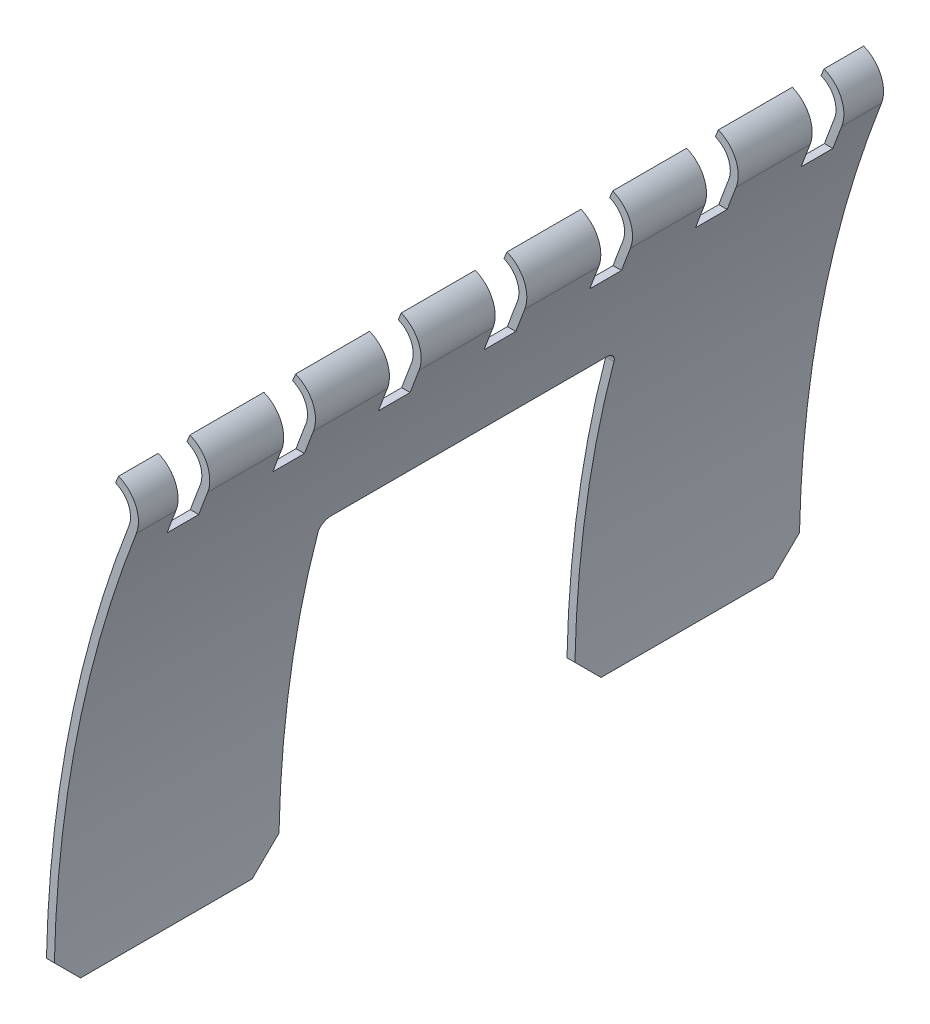
SolidWorks part; units mm, degrees
ref_plane "Front Plane" through (0, 0, 0) normal (0, 0, 1) x (1, 0, 0)
ref_plane "Top Plane" through (0, 0, 0) normal (0, 1, 0) x (1, 0, 0)
ref_plane "Right Plane" through (0, 0, 0) normal (1, 0, 0) x (0, 0, -1)
sketch "Sketch1" plane through (0, 0, 0) normal (0, 0, 1) x (1, 0, 0)
  line L0 (-229.8, 0) -> (-231.3, 0)
  line L1 (0, 0) -> (-315.3117, 122.3014) construction
  arc A0 (-214.248, 83.1013) -> (-229.8, 0) centre (0, 0) ccw
  arc A1 (-215.6465, 83.6438) -> (-231.3, 0) centre (0, 0) ccw
  arc A2 (-217.6012, 90.837) -> (-218.1747, 89.4508) centre (0, 0) ccw
  arc A3 (-214.248, 83.1013) -> (-217.6012, 90.837) centre (-219.842, 85.2711) ccw
  circle A4 centre (0, 0) radius 231.3 construction
  circle A5 centre (0, 0) radius 229.8 construction
  arc A6 (-215.6465, 83.6438) -> (-218.1747, 89.4508) centre (-219.842, 85.2711) ccw
  circle A8 centre (-219.842, 85.2711) radius 4.5 construction
  circle A9 centre (-219.842, 85.2711) radius 6 construction
  point P4 (219.7588, 67.187)
  point P5 (231.3, 0)
  point P8 (-219.842, 85.2711)
  point P19 (-215.342, 85.2711)
  point P21 (-214.1041, 87.0253)
  dimension "D1" = 459.6
  dimension "D4" = 235.8
  dimension "D5" = 12
  dimension "D3" = 21.2
  dimension "D2" = 1.5
extrude "Boss-Extrude1" add sketch "Sketch1" along normal mid plane 141
sketch "Sketch2" plane through (0, 0, 0) normal (0, 0, 1) x (1, 0, 0)
  line L0 (-231.3, 0) -> (-229.8, 0) construction
  line L1 (-256.8852, 60) -> (-194.6945, 60)
  line L2 (-256.8852, 60) -> (-256.8852, -22.2291)
  line L3 (-256.8852, -22.2291) -> (-194.6945, -22.2291)
  line L4 (-194.6945, 60) -> (-194.6945, -22.2291)
  dimension "D1" = 60
extrude "Cut-Extrude1" cut sketch "Sketch2" against normal mid plane 56
fillet "Fillet1" radius 2 2 edges at (-222.6056, 60, 28) (-222.6056, 60, -28)
chamfer "Chamfer2" distance 5 angle 45 4 edges at (-230.55, 0, -28) (-230.55, 0, -70.5) (-230.55, 0, 70.5) (-230.55, 0, 28)
sketch "Sketch3" plane through (0, 0, 0) normal (1, 0, 0) x (0, 0, -1)
  line L0 (70.5, 5) -> (70.5, 83.1013) construction
  line L1 (57, 90.837) -> (63, 90.837)
  line L2 (57, 90.837) -> (57, 78.637)
  line L3 (57, 78.637) -> (63, 78.637)
  line L4 (63, 90.837) -> (63, 78.637)
  line L5 (-70.5, 90.837) -> (70.5, 90.837) construction
  line L6 (37, 78.637) -> (43, 78.637)
  line L7 (37, 90.837) -> (37, 78.637)
  line L8 (43, 90.837) -> (43, 78.637)
  line L9 (37, 90.837) -> (43, 90.837)
  line L10 (17, 78.637) -> (23, 78.637)
  line L11 (17, 90.837) -> (17, 78.637)
  line L12 (23, 90.837) -> (23, 78.637)
  line L13 (17, 90.837) -> (23, 90.837)
  line L14 (-3, 78.637) -> (3, 78.637)
  line L15 (-3, 90.837) -> (-3, 78.637)
  line L16 (3, 90.837) -> (3, 78.637)
  line L17 (-3, 90.837) -> (3, 90.837)
  line L18 (-23, 78.637) -> (-17, 78.637)
  line L19 (-23, 90.837) -> (-23, 78.637)
  line L20 (-17, 90.837) -> (-17, 78.637)
  line L21 (-23, 90.837) -> (-17, 90.837)
  line L22 (-43, 78.637) -> (-37, 78.637)
  line L23 (-43, 90.837) -> (-43, 78.637)
  line L24 (-37, 90.837) -> (-37, 78.637)
  line L25 (-43, 90.837) -> (-37, 90.837)
  line L26 (-63, 78.637) -> (-57, 78.637)
  line L27 (-63, 90.837) -> (-63, 78.637)
  line L28 (-57, 90.837) -> (-57, 78.637)
  line L29 (-63, 90.837) -> (-57, 90.837)
  dimension "D1" = 7.5
  dimension "D2" = 12.2
  dimension "D3" = 6
  dimension "D5" = 20
  dimension "D4" = 7
extrude "Cut-Extrude2" cut sketch "Sketch3" against normal through all
